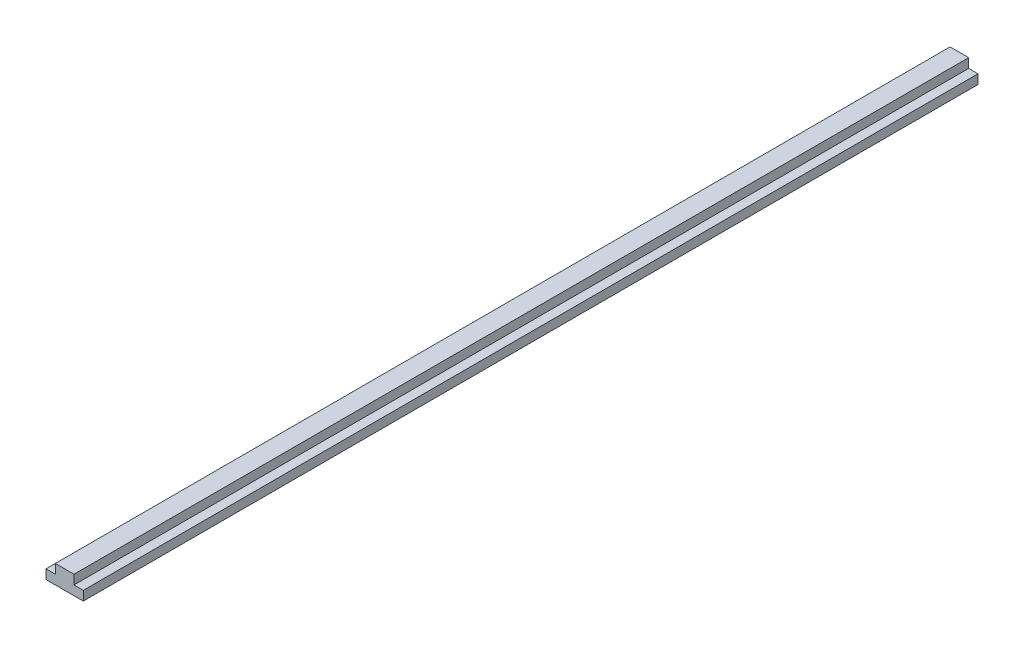
from build123d import *

# Parameters (mm, degrees)
BOSS_EXTRUDE1_DEPTH = 480


with BuildPart() as part:
    # Sketch1 → Boss-Extrude1 (new body)
    with BuildSketch(Plane.XY):
        Polygon((5, 5), (5, 10), (15, 10), (15, 5), (20, 5), (20, 0), (0, 0), (0, 5), align=None)
    extrude(amount=BOSS_EXTRUDE1_DEPTH)


solid = part.part
